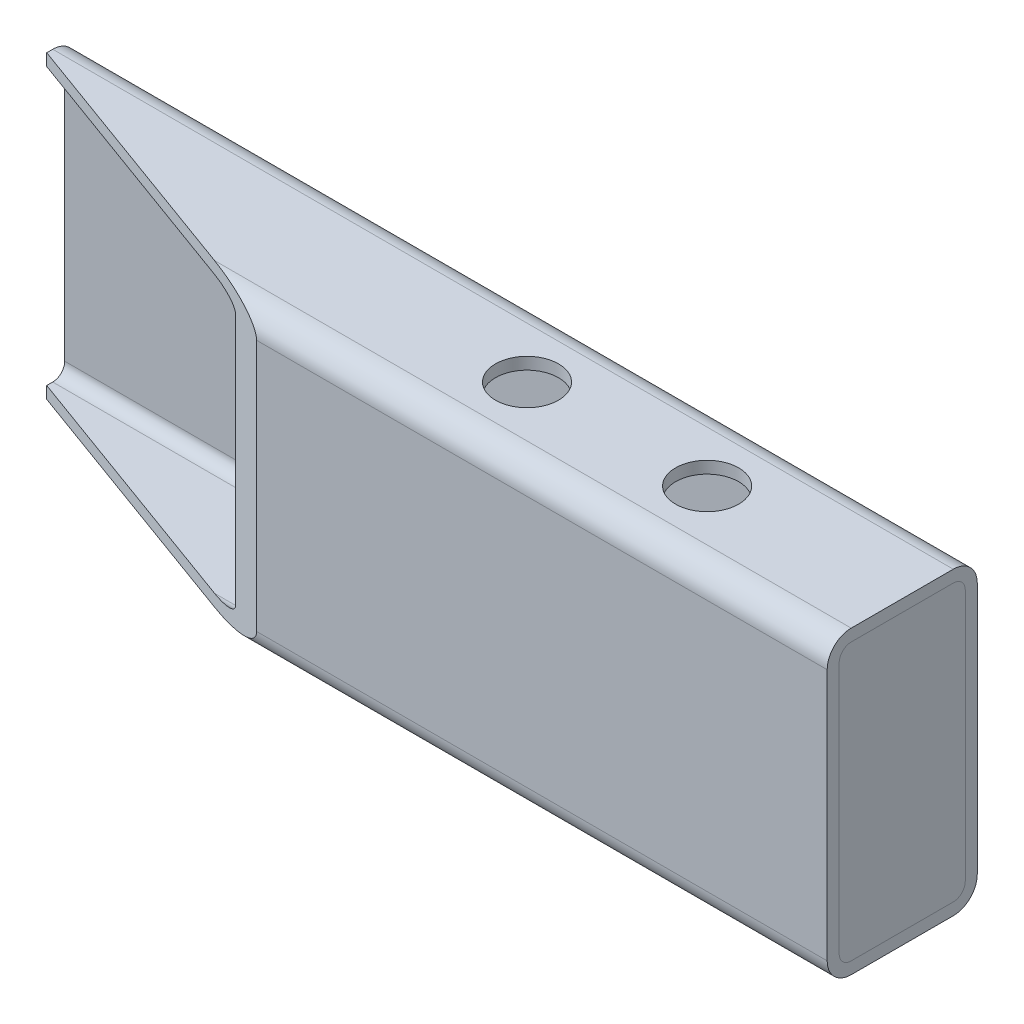
SolidWorks part; units mm, degrees
material "普通碳钢"
ref_plane "前视基准面" through (0, 0, 0) normal (0, 0, 1) x (1, 0, 0)
ref_plane "上视基准面" through (0, 0, 0) normal (0, 1, 0) x (1, 0, 0)
ref_plane "右视基准面" through (0, 0, 0) normal (1, 0, 0) x (0, 0, -1)
sketch3d "3D草图1"
  line L0 (0, 0, 0) -> (300, 0, 0)
  dimension "D1" = 300
other "矩形管 100 X 50 X 4(1)"
ref_plane "基准面1" through (0, 0, 0) normal (1, 0, 0) x (0, 0, -1)
sketch "Sketch1" plane through (0, 0, 0) normal (1, 0, 0) x (0, 0, -1)
  line L0 (-17, -46) -> (17, -46)
  line L1 (-21, -42) -> (-21, 42)
  line L2 (17, 46) -> (-17, 46)
  line L3 (21, 42) -> (21, -42)
  line L4 (-17, -50) -> (17, -50)
  line L5 (-25, -42) -> (-25, 42)
  line L6 (17, 50) -> (-17, 50)
  line L7 (25, 42) -> (25, -42)
  arc A0 (25, 42) -> (17, 50) centre (17, 42) ccw
  arc A1 (17, -50) -> (25, -42) centre (17, -42) ccw
  arc A2 (-25, -42) -> (-17, -50) centre (-17, -42) ccw
  arc A3 (-17, 50) -> (-25, 42) centre (-17, 42) ccw
  arc A4 (-17, 46) -> (-21, 42) centre (-17, 42) ccw
  arc A5 (21, 42) -> (17, 46) centre (17, 42) ccw
  arc A6 (17, -46) -> (21, -42) centre (17, -42) ccw
  arc A7 (-21, -42) -> (-17, -46) centre (-17, -42) ccw
  point P0 (0, 50)
  point P1 (25, 0)
  point P2 (0, -50)
  point P3 (-25, 0)
  point P4 (-25, 50)
  point P5 (25, 50)
  point P6 (25, -50)
  point P7 (-25, -50)
  point P8 (0, 0)
  point P33 (0, 0)
  dimension "D1" = 8
  dimension "Thickness" = 4
  dimension "V_leg" = 100
  dimension "H_leg" = 50
sketch "草图2" plane through (0, -50, 0) normal (0, -1, 0) x (1, 0, 0)
  line L0 (0, -15) -> (109.8991, 25)
  line L1 (0, 17) -> (0, -17) construction
  line L2 (300, 25) -> (0, 25) construction
  line L3 (109.8991, 25) -> (0, 25)
  line L4 (0, 25) -> (0, -15)
  line L5 (300, 0) -> (0, 0) construction
  line L6 (300, 17) -> (300, -17) construction
  circle A0 centre (235, 0) radius 10.5
  circle A1 centre (175, 0) radius 10.5
  dimension "D3" = 21
  dimension "D4" = 21
  dimension "D1" = 40
  dimension "D2" = 20
  dimension "D5" = 65
  dimension "D6" = 60
extrude "切除-拉伸1" cut sketch "草图2" against normal up to surface (100 mm away) up to face at (150, 50, 0)
sketch "草图3" plane through (300, 0, 0) normal (1, 0, 0) x (0, 0, -1)
  line L0 (17, 46) -> (-17, 46) construction
  line L1 (-17, 46) -> (17, 46)
  line L2 (-21, 42) -> (-21, -42)
  line L3 (-17, -46) -> (17, -46)
  line L4 (21, 42) -> (21, -42)
  line L5 (21, -42) -> (21, 42) construction
  line L6 (-21, 42) -> (-21, -42) construction
  line L7 (-17, -46) -> (17, -46) construction
  arc A1 (-21, -42) -> (-17, -46) centre (-17, -42) ccw
  arc A2 (17, -46) -> (21, -42) centre (17, -42) ccw
  arc A3 (17, 46) -> (21, 42) centre (17, 42) cw
  arc A4 (-17, 46) -> (-21, 42) centre (-17, 42) ccw
  dimension "D1" = 4
extrude "凸台-拉伸1" add sketch "草图3" against normal blind 25 separate body
